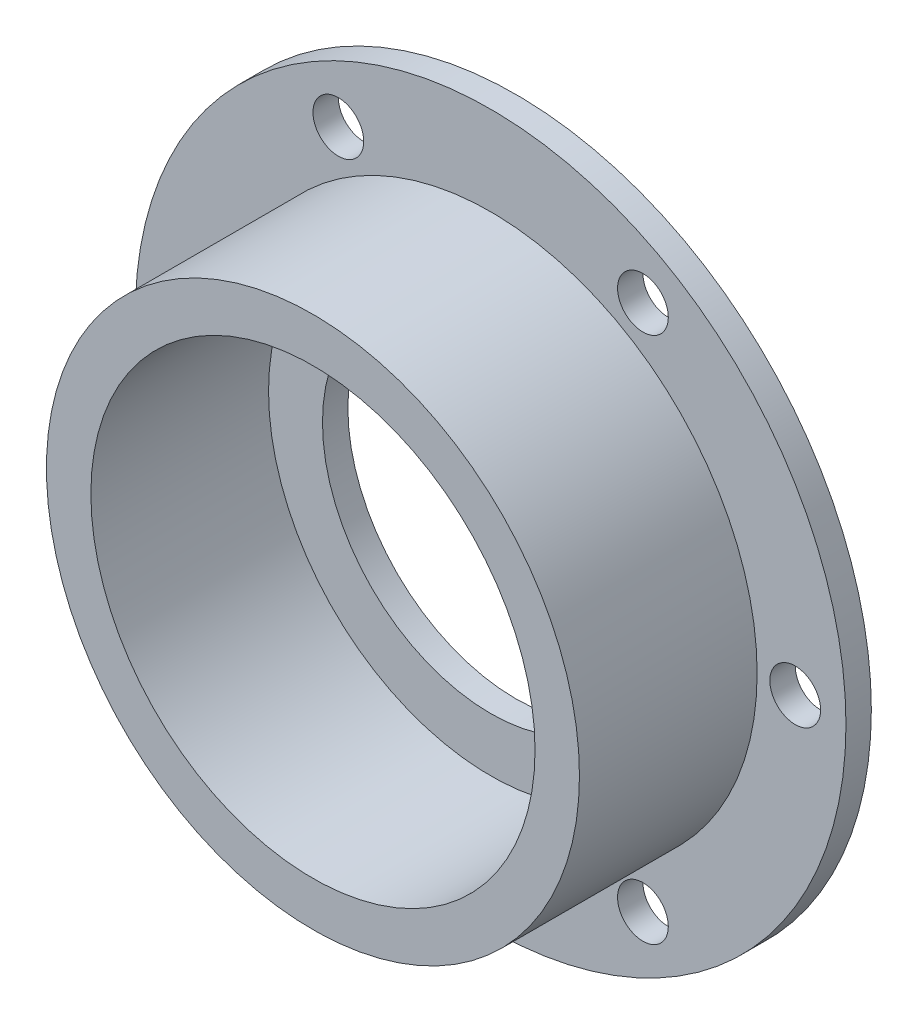
SolidWorks part; units mm, degrees
ref_plane "前视基准面" through (0, 0, 0) normal (0, 0, 1) x (1, 0, 0)
ref_plane "上视基准面" through (0, 0, 0) normal (0, 1, 0) x (1, 0, 0)
ref_plane "右视基准面" through (0, 0, 0) normal (1, 0, 0) x (0, 0, -1)
sketch "草图1" plane through (0, 0, 0) normal (0, 0, 1) x (1, 0, 0)
  circle A0 centre (0, 0) radius 280
extrude "凸台-拉伸1" add sketch "草图1" along normal blind 20
sketch "草图2" plane through (0, 0, 0) normal (0, 0, 1) x (1, 0, 0)
  circle A0 centre (0, 0) radius 210
extrude "凸台-拉伸2" add sketch "草图2" along normal blind 160
sketch3d "3D草图1"
  point P0 (38.1779, 59.288, 160)
ref_plane "基准面1" through (0, 0, 160) normal (0, 0, 1) x (1, 0, 0)
sketch "草图3" plane through (0, 0, 160) normal (0, 0, 1) x (1, 0, 0)
  circle A0 centre (0, 0) radius 175
extrude "切除-拉伸1" cut sketch "草图3" against normal up to surface (140 mm away) up to face at (210, 0, 20)
sketch "草图4" plane through (0, 0, 0) normal (0, 0, 1) x (1, 0, 0)
  circle A1 centre (240, 0) radius 20
  circle A2 centre (-240, 0) radius 20
  circle A3 centre (-120, 207.8461) radius 20
  circle A4 centre (120, 207.8461) radius 20
  circle A5 centre (-120, -207.8461) radius 20
  circle A6 centre (120, -207.8461) radius 20
extrude "切除-拉伸3" cut sketch "草图4" along normal blind 20
sketch "草图5" plane through (0, 0, 0) normal (0, 0, 1) x (1, 0, 0)
  circle A0 centre (0, 0) radius 132.5
extrude "切除-拉伸4" cut sketch "草图5" along normal blind 20
